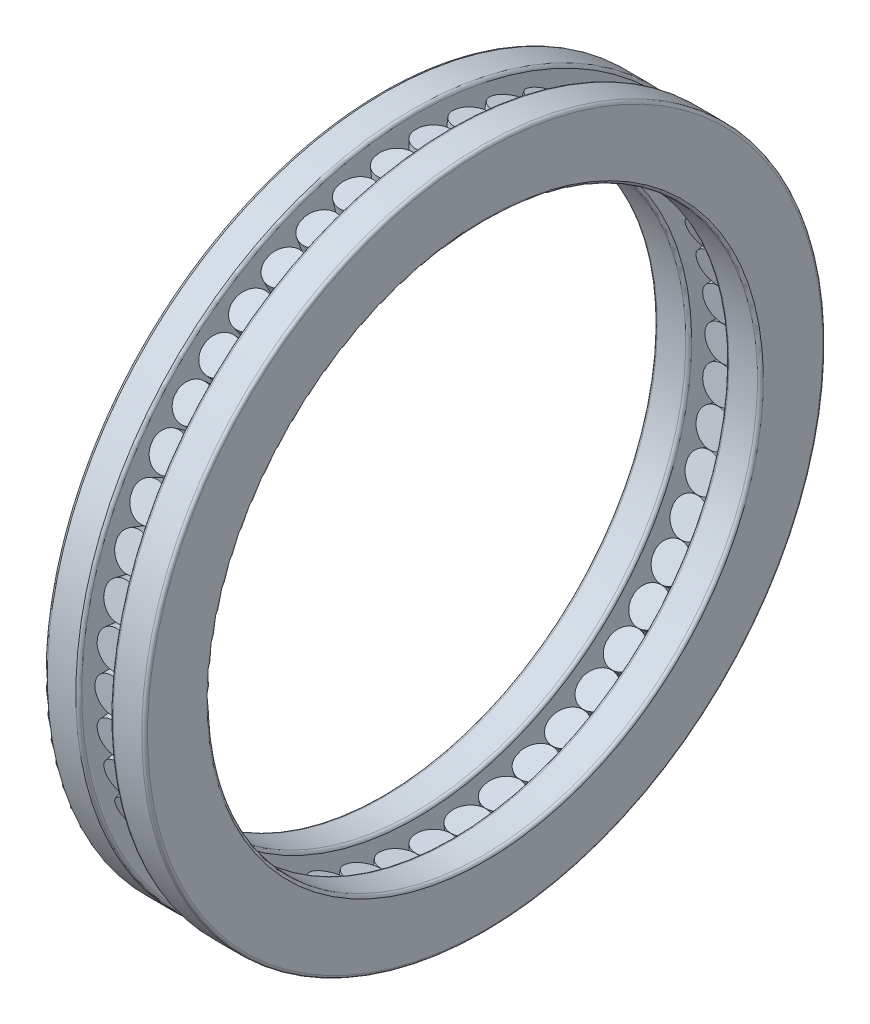
from build123d import *

# Parameters (mm, degrees)
SKETCH1_W               = 33.5
SKETCH1_H               = 17.666666667
SKETCH2_W               = 16.75
SKETCH2_H               = 8.933333334
SKETCH3_W               = 33.5
SKETCH3_H               = 17.666666666
CIRCULAR_PATTERN1_COUNT = 52
FILLET1_R               = 1.5


with BuildPart() as part:
    # Sketch1 → Revolve1 (revolve)
    with BuildSketch(Plane(origin=(-7.03002736, 10.46997264, 0), x_dir=(0, 1, 0), z_dir=(0, 0, 1))):
        with Locations((-167.21997264, 1.803305974)):
            Rectangle(SKETCH1_W, SKETCH1_H)
    revolve(axis=Axis((-25.185294118, 0, 0), (1, 0, 0)))

    # Sketch2 → Revolve2 (revolve)
    with BuildSketch(Plane(origin=(1.570880833, -3.029119167, 0), x_dir=(0, -1, 0), z_dir=(0, 0, 1))):
        with Locations((-159.779119167, 11.729119167)):
            Rectangle(SKETCH2_W, SKETCH2_H)
    revolve2 = revolve(axis=Axis((8.833333333, 16.546140247, 0), (0, -1, 0)))

    # Sketch3 → Revolve3 (revolve)
    with BuildSketch(Plane(origin=(-8.782998936, 8.717001064, 0), x_dir=(0, 1, 0), z_dir=(0, 0, 1))):
        with Locations((-166.967001064, -35.282998936)):
            Rectangle(SKETCH3_W, SKETCH3_H)
    revolve(axis=Axis((-15.612745098, 0, 0), (1, 0, 0)))

    # Circular-Pattern1: Revolve2 ×52 about axis
    circular_pattern1_axis = Axis((0, 0, 0), (1, 0, 0))
    for i in range(1, CIRCULAR_PATTERN1_COUNT):
        add(revolve2.rotate(circular_pattern1_axis, i * 360 / CIRCULAR_PATTERN1_COUNT))

    # Fillet1
    fillet1_edges = [part.edges().sort_by_distance(p)[0] for p in [
        (17.666666667, 175, 0),
        (35.333333333, 175, 0),
        (35.333333333, 141.5, 0),
        (17.666666667, 141.5, 0),
        (0, 173.5, 0),
        (0, 140, 0),
        (-17.666666667, 140, 0),
        (-17.666666667, 173.5, 0),
    ]]
    fillet(fillet1_edges, radius=FILLET1_R)


solid = part.part
